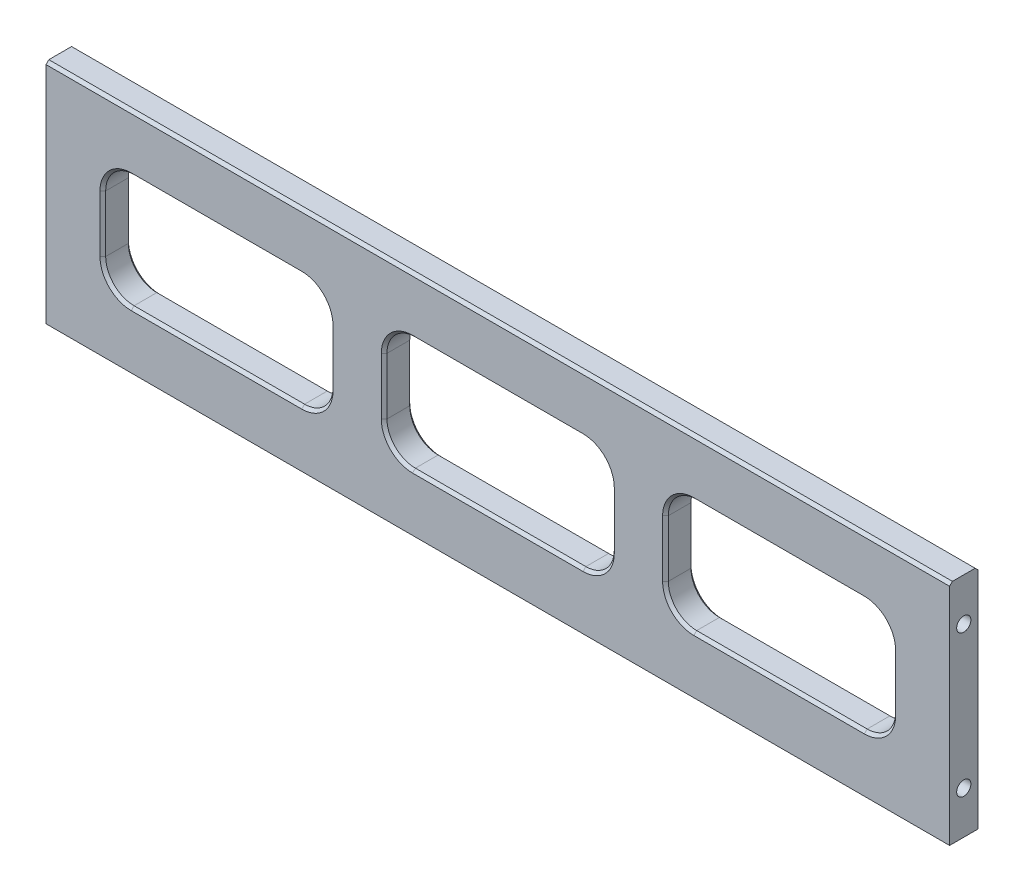
from build123d import *

# Parameters (mm, degrees)
SKETCH_1_W                = 318
SKETCH_1_H                = 80
EXTRUDE_1_DEPTH           = 10
SKETCH_2_W                = 80
SKETCH_2_H                = 40
CUT_EXTRUDE_1_DEPTH       = 189.098378515
SKETCH_3_W                = 80
SKETCH_3_H                = 40
CUT_EXTRUDE_2_DEPTH       = 189.098378515
SKETCH_4_W                = 80
SKETCH_4_H                = 40
CUT_EXTRUDE_3_DEPTH       = 189.098378515
HOLE_WIZARD_5_0_5_1_D     = 5
HOLE_WIZARD_5_0_5_1_DEPTH = 15
HOLE_WIZARD_5_0_5_1_TIP   = 1.502151548
HOLE_WIZARD_5_0_5_2_D     = 5
HOLE_WIZARD_5_0_5_2_DEPTH = 15
HOLE_WIZARD_5_0_5_2_TIP   = 1.502151548
HOLE_WIZARD_5_0_5_3_D     = 5
HOLE_WIZARD_5_0_5_3_DEPTH = 15
HOLE_WIZARD_5_0_5_3_TIP   = 1.502151548
FILLET_1_R                = 10
CHAMFER_1_SIZE            = 1


with BuildPart() as part:
    # 草图1 → 凸台-拉伸1 (new body)
    with BuildSketch(Plane.XY.offset(10)):
        with Locations((0, -60)):
            Rectangle(SKETCH_1_W, SKETCH_1_H)
    extrude(amount=-EXTRUDE_1_DEPTH)

    # 草图2 → 切除-拉伸1 (cut, through all)
    with BuildSketch(Plane.XY.offset(10)):
        with Locations((0, -60)):
            Rectangle(SKETCH_2_W, SKETCH_2_H)
    extrude(amount=-CUT_EXTRUDE_1_DEPTH, mode=Mode.SUBTRACT)

    # 草图3 → 切除-拉伸2 (cut, through all)
    with BuildSketch(Plane.XY.offset(10)):
        with Locations((99, -60)):
            Rectangle(SKETCH_3_W, SKETCH_3_H)
    extrude(amount=-CUT_EXTRUDE_2_DEPTH, mode=Mode.SUBTRACT)

    # 草图4 → 切除-拉伸3 (cut, through all)
    with BuildSketch(Plane(origin=(0, 0, 0), x_dir=(-1, 0, 0), z_dir=(0, 0, -1))):
        with Locations((99, -60)):
            Rectangle(SKETCH_4_W, SKETCH_4_H)
    extrude(amount=-CUT_EXTRUDE_3_DEPTH, mode=Mode.SUBTRACT)

    # Ø5.0 (5) 直径孔1
    with Locations(Plane.ZY.offset(159)):
        with Locations((5, -35), (5, -85)):
            Hole(HOLE_WIZARD_5_0_5_1_D / 2, depth=HOLE_WIZARD_5_0_5_1_DEPTH)
            with Locations((0, 0, -(HOLE_WIZARD_5_0_5_1_DEPTH + HOLE_WIZARD_5_0_5_1_TIP / 2))):  # 118° drill point
                Cone(0, HOLE_WIZARD_5_0_5_1_D / 2, HOLE_WIZARD_5_0_5_1_TIP, mode=Mode.SUBTRACT)

    # Ø5.0 (5) 直径孔2
    with Locations(Plane(origin=(159, 0, 0), x_dir=(0, 0, -1), z_dir=(1, 0, 0))):
        with Locations((-5, -35), (-5, -85)):
            Hole(HOLE_WIZARD_5_0_5_2_D / 2, depth=HOLE_WIZARD_5_0_5_2_DEPTH)
            with Locations((0, 0, -(HOLE_WIZARD_5_0_5_2_DEPTH + HOLE_WIZARD_5_0_5_2_TIP / 2))):  # 118° drill point
                Cone(0, HOLE_WIZARD_5_0_5_2_D / 2, HOLE_WIZARD_5_0_5_2_TIP, mode=Mode.SUBTRACT)

    # Ø5.0 (5) 直径孔3
    with Locations(Plane(origin=(0, -100, 0), x_dir=(-1, 0, 0), z_dir=(0, -1, 0))):
        with Locations((121.5, -5), (40.5, -5), (-40.5, -5), (-121.5, -5)):
            Hole(HOLE_WIZARD_5_0_5_3_D / 2, depth=HOLE_WIZARD_5_0_5_3_DEPTH)
            with Locations((0, 0, -(HOLE_WIZARD_5_0_5_3_DEPTH + HOLE_WIZARD_5_0_5_3_TIP / 2))):  # 118° drill point
                Cone(0, HOLE_WIZARD_5_0_5_3_D / 2, HOLE_WIZARD_5_0_5_3_TIP, mode=Mode.SUBTRACT)

    # 圆角1
    fillet_1_edges = [part.edges().sort_by_distance(p)[0] for p in [
        (40, -80, 5),
        (-40, -80, 5),
        (-40, -40, 5),
        (40, -40, 5),
        (139, -80, 5),
        (59, -80, 5),
        (59, -40, 5),
        (139, -40, 5),
        (-59, -40, 5),
        (-139, -40, 5),
        (-139, -80, 5),
        (-59, -80, 5),
    ]]
    fillet(fillet_1_edges, radius=FILLET_1_R)

    # 倒角1
    chamfer_1_edges = [part.edges().sort_by_distance(p)[0] for p in [
        (0, -40, 10),
        (0, -40, 0),
        (40, -60, 10),
        (40, -60, 0),
        (99, -40, 10),
        (99, -40, 0),
        (139, -60, 10),
        (139, -60, 0),
        (0, -80, 10),
        (0, -80, 0),
        (-40, -60, 10),
        (-40, -60, 0),
        (99, -80, 10),
        (99, -80, 0),
        (-99, -40, 0),
        (-99, -40, 10),
        (-139, -60, 0),
        (-139, -60, 10),
        (59, -60, 10),
        (59, -60, 0),
        (-59, -60, 0),
        (-59, -60, 10),
        (-99, -80, 0),
        (-99, -80, 10),
        (37.071067812, -42.928932188, 10),
        (37.071067812, -42.928932188, 0),
        (136.071067812, -42.928932188, 10),
        (136.071067812, -42.928932188, 0),
        (-37.071067812, -77.071067812, 10),
        (-37.071067812, -77.071067812, 0),
        (136.071067812, -77.071067812, 10),
        (136.071067812, -77.071067812, 0),
        (-136.071067812, -42.928932188, 0),
        (-136.071067812, -42.928932188, 10),
        (61.928932188, -42.928932188, 10),
        (61.928932188, -42.928932188, 0),
        (37.071067812, -77.071067812, 10),
        (37.071067812, -77.071067812, 0),
        (-61.928932188, -42.928932188, 0),
        (-61.928932188, -42.928932188, 10),
        (-37.071067812, -42.928932188, 10),
        (-37.071067812, -42.928932188, 0),
        (-61.928932188, -77.071067812, 0),
        (-61.928932188, -77.071067812, 10),
        (-136.071067812, -77.071067812, 0),
        (-136.071067812, -77.071067812, 10),
        (61.928932188, -77.071067812, 10),
        (61.928932188, -77.071067812, 0),
        (0, -20, 0),
        (0, -20, 10),
    ]]
    chamfer(chamfer_1_edges, length=CHAMFER_1_SIZE)


solid = part.part
